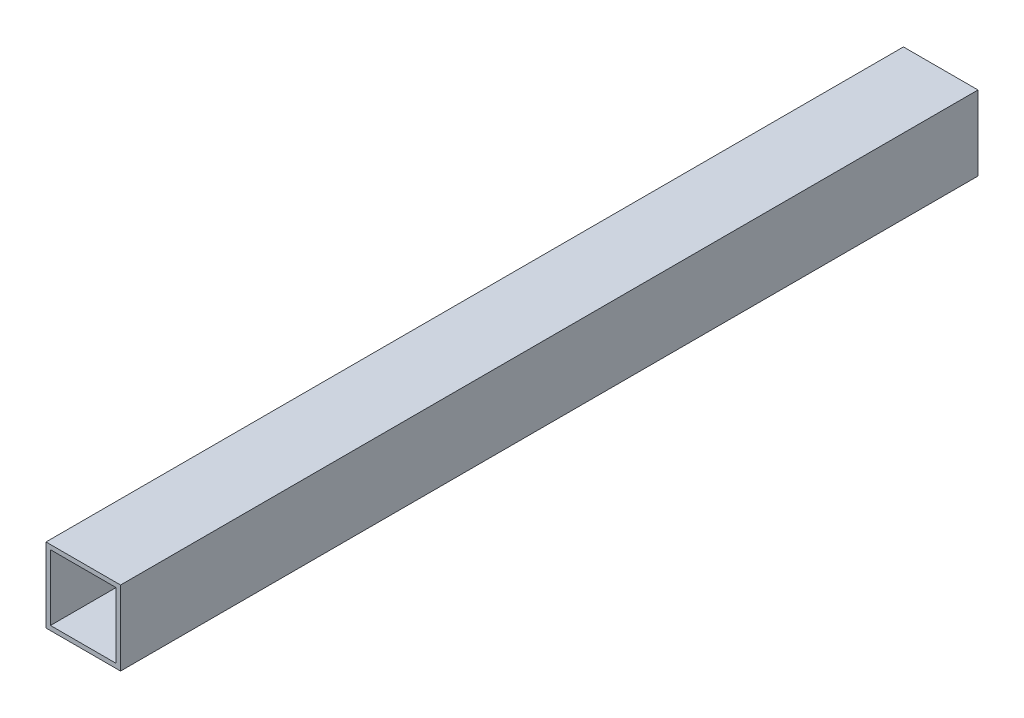
SolidWorks part; units mm, degrees
ref_plane "前视基准面" through (0, 0, 0) normal (0, 0, 1) x (1, 0, 0)
ref_plane "上视基准面" through (0, 0, 0) normal (0, 1, 0) x (1, 0, 0)
ref_plane "右视基准面" through (0, 0, 0) normal (1, 0, 0) x (0, 0, -1)
sketch "草图1" plane through (0, 0, 0) normal (0, 0, 1) x (1, 0, 0)
  line L0 (0, 0) -> (0, 50)
  line L1 (0, 50) -> (50, 50)
  line L2 (50, 50) -> (50, 0)
  line L3 (50, 0) -> (0, 0)
  line L4 (3, 3) -> (3, 47)
  line L5 (3, 47) -> (47, 47)
  line L6 (47, 47) -> (47, 3)
  line L7 (47, 3) -> (3, 3)
  dimension "D1" = 3
extrude "凸台-拉伸1" add sketch "草图1" along normal blind 600
sketch "草图2" plane through (0, 0, 600) normal (0, 0, 1) x (1, 0, 0)
  line L4 (47, 3) -> (47, 47)
  line L5 (47, 47) -> (3, 47)
  line L6 (3, 47) -> (3, 3)
  line L7 (3, 3) -> (47, 3)
  line L8 (0, 0) -> (50, 0)
  line L9 (50, 0) -> (50, 50)
  line L10 (50, 50) -> (0, 50)
  line L11 (0, 50) -> (0, 0)
  line L12 (0, 0) -> (50, 0)
  line L13 (50, 0) -> (50, 50)
  line L14 (50, 50) -> (0, 50)
  line L15 (0, 50) -> (0, 0)
  dimension "D1" = 0
extrude "切除-拉伸1" cut sketch "草图2" against normal blind 25
